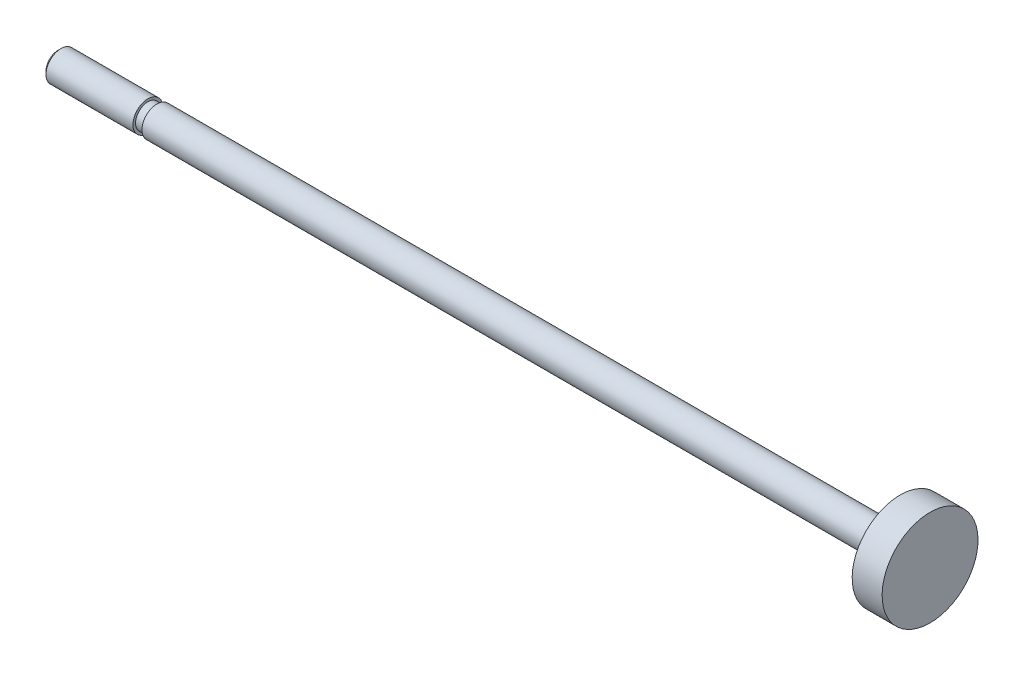
from build123d import *


with BuildPart() as part:
    # Sketch1 → Revolve1 (revolve)
    with BuildSketch(Plane.XY, mode=Mode.PRIVATE) as revolve1_sk:
        Polygon((0, 0), (0, 2.0095), (0.4905, 2.5), (15, 2.5), (15, 2.067), (16.5, 2.067), (16.5, 2.5), (140.5, 2.5), (140.5, 8), (145.5, 8), (145.5, 0), align=None)
    revolve(revolve1_sk.sketch.rotate(Axis((145.5, 0, 0), (-1, 0, 0)), 180), axis=Axis((145.5, 0, 0), (-1, 0, 0)))


solid = part.part
